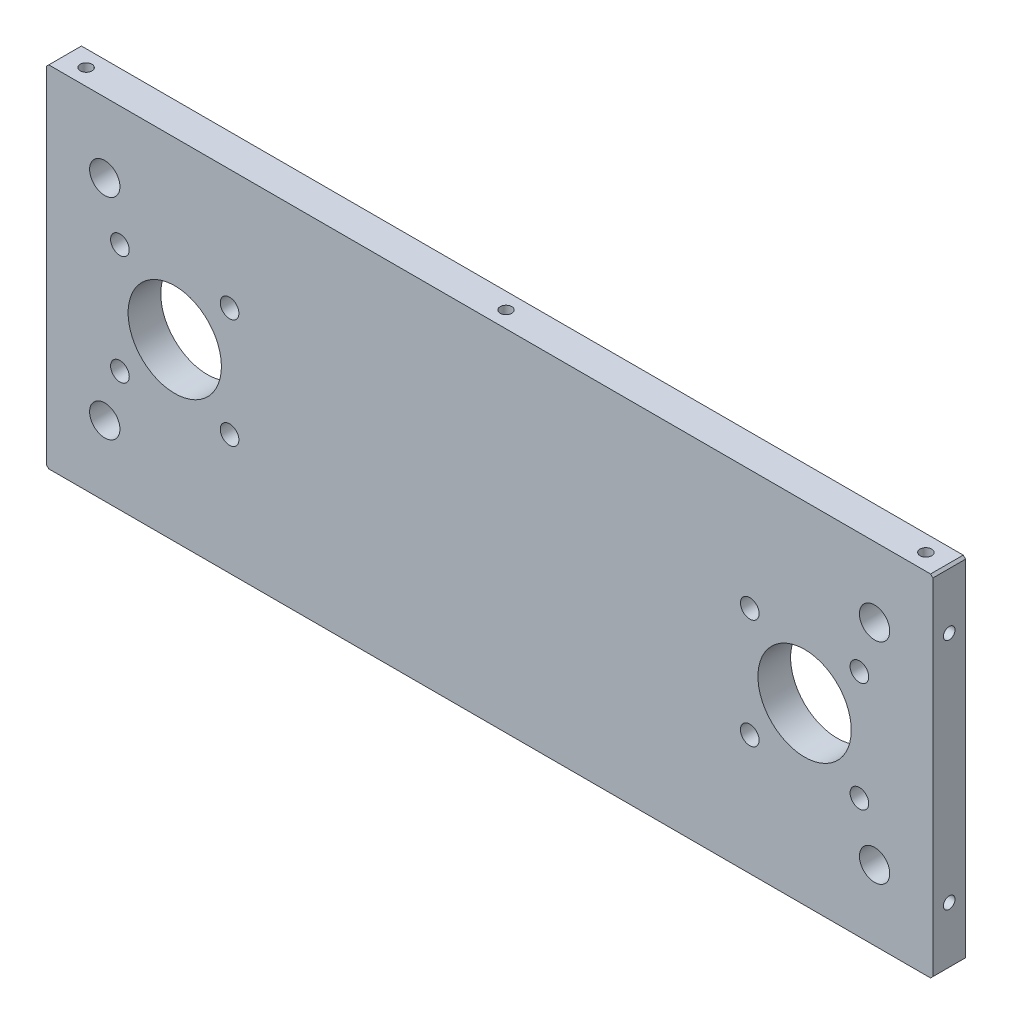
SolidWorks part; units mm, degrees
material "普通碳钢"
ref_plane "Front Plane" through (0, 0, 0) normal (0, 0, 1) x (1, 0, 0)
ref_plane "Top Plane" through (0, 0, 0) normal (0, 1, 0) x (1, 0, 0)
ref_plane "Right Plane" through (0, 0, 0) normal (1, 0, 0) x (0, 0, -1)
sketch "Sketch1" plane through (0, 0, 0) normal (0, 0, 1) x (1, 0, 0)
  line L1 (0, 0) -> (380, 0)
  line L2 (0, 0) -> (0, 150)
  line L3 (0, 150) -> (380, 150)
  line L4 (380, 0) -> (380, 150)
  dimension "D1" = 380
  dimension "D2" = 150
extrude "Boss-Extrude1" add sketch "Sketch1" along normal blind 14
chamfer "Chamfer1" distance 1 angle 45 4 edges at (0, 0, 7) (0, 150, 7) (380, 0, 7) (380, 150, 7)
sketch "Sketch2" plane through (0, 0, 14) normal (0, 0, 1) x (1, 0, 0)
  line L0 (0, 75) -> (55, 75) construction
  line L1 (0, 149) -> (0, 1) construction
  line L2 (55, 75) -> (325, 75) construction
  line L3 (190, 75) -> (190, 150) construction
  line L4 (379, 150) -> (1, 150) construction
  circle A0 centre (55, 75) radius 20
  circle A1 centre (325, 75) radius 20
  dimension "D1" = 40
  dimension "D2" = 270
extrude "Cut-Extrude1" cut sketch "Sketch2" against normal through all
hole_wizard "Ø8.0 (8) Diameter Hole1" positions "3DSketch1" profile "Sketch3" hole size "Ø8.0" standard "GB" end condition through all
sketch3d "3DSketch1"
  line L0 (31.5, 98.5, 14) -> (78.5, 98.5, 14) construction
  line L1 (78.5, 98.5, 14) -> (78.5, 51.5, 14) construction
  line L2 (78.5, 51.5, 14) -> (31.5, 51.5, 14) construction
  line L3 (31.5, 51.5, 14) -> (31.5, 98.5, 14) construction
  line L5 (31.5, 75, 14) -> (55, 75, 14) construction
  line L6 (55, 75, 0) -> (55, 75, 14) construction
  line L7 (55, 75, 14) -> (55, 98.5, 14) construction
  point P0 (31.5, 98.5, 14)
  point P2 (78.5, 98.5, 14)
  point P4 (78.5, 51.5, 14)
  point P6 (31.5, 51.5, 14)
  dimension "D1" = 47
  dimension "D2" = 47
sketch "Sketch3" plane through (31.5, 98.5, 14) normal (1, 0, 0) x (0, -1, 0)
  line L0 (0, 0) -> (0, 14)
  line L1 (0, 14) -> (4, 14)
  line L2 (4, 14) -> (4, 0)
  line L5 (4, 0) -> (0, 0)
  line L11 (0, -6.35) -> (0, 107.95) construction
  dimension "通孔孔直径" = 8
  dimension "通孔孔深度" = 14
pattern_linear "LPattern1" count 2 spacing 270 along (1, 0, 0) of "Ø8.0 (8) Diameter Hole1"
hole_wizard "Ø13.0 (13) Diameter Hole1" positions "3DSketch2" profile "Sketch4" hole size "Ø13.0" standard "GB" end condition through all
sketch3d "3DSketch2"
  line L0 (355, 120, 0) -> (355, 30, 0) construction
  line L1 (355, 30, 0) -> (25, 30, 0) construction
  line L2 (25, 30, 0) -> (25, 120, 0) construction
  line L3 (25, 120, 0) -> (355, 120, 0) construction
  line L5 (355, 75, 0) -> (380, 75, 0) construction
  line L6 (380, 1, 0) -> (380, 149, 0) construction
  line L8 (190, 120, 0) -> (190, 150, 0) construction
  line L9 (379, 150, 0) -> (1, 150, 0) construction
  point P0 (355, 120, 0)
  point P2 (355, 30, 0)
  point P4 (25, 30, 0)
  point P6 (25, 120, 0)
  dimension "D1" = 330
  dimension "D2" = 90
sketch "Sketch4" plane through (355, 120, 0) normal (1, 0, 0) x (0, 1, 0)
  line L0 (0, 0) -> (0, 14)
  line L1 (0, 14) -> (6.5, 14)
  line L2 (6.5, 14) -> (6.5, 0)
  line L5 (6.5, 0) -> (0, 0)
  line L11 (0, -6.35) -> (0, 107.95) construction
  dimension "通孔孔直径" = 13
  dimension "通孔孔深度" = 14
hole_wizard "M6 Tapped Hole1" positions "Sketch5" profile "Sketch6" tap size "M6" standard "GB"
sketch "Sketch5" plane through (0, 0, 0) normal (0, -1, 0) x (-1, 0, 0)
  line L0 (-190, 0) -> (-190, -7) construction
  line L1 (-1, 0) -> (-379, 0) construction
  point P0 (-370, -7)
  point P2 (-190, -7)
  point P4 (-10, -7)
  dimension "D1" = 7
  dimension "D2" = 360
sketch "Sketch6" plane through (370, 0, 7) normal (1, 0, 0) x (0, 0, -1)
  line L0 (0, 0) -> (0, 16.5022)
  line L1 (0, 16.5022) -> (2.5, 15)
  line L2 (2.5, 15) -> (2.5, 0)
  line L5 (2.5, 0) -> (0, 0)
  line L10 (0, 16.5022) -> (-2.5, 15) construction
  line L11 (0, -6.35) -> (0, 107.95) construction
  dimension "螺纹孔钻头直径" = 5
  dimension "螺纹孔钻头深度" = 15
  dimension "导头角度" = 118
cosmetic thread "Cosmetic Thread1" parameters "D1"=12, "D2"=6
cosmetic thread "Cosmetic Thread2" parameters "D1"=12, "D2"=6
cosmetic thread "Cosmetic Thread3" parameters "D1"=12, "D2"=6
hole_wizard "M6 Tapped Hole2" positions "Sketch7" profile "Sketch8" tap size "M6" standard "GB"
sketch "Sketch7" plane through (0, 150, 0) normal (0, 1, 0) x (1, 0, 0)
  point P0 (370, -7)
  point P3 (190, -7)
  point P6 (10, -7)
sketch "Sketch8" plane through (370, 150, 7) normal (1, 0, 0) x (0, 0, 1)
  line L0 (0, 0) -> (0, 16.5022)
  line L1 (0, 16.5022) -> (2.5, 15)
  line L2 (2.5, 15) -> (2.5, 0)
  line L5 (2.5, 0) -> (0, 0)
  line L10 (0, 16.5022) -> (-2.5, 15) construction
  line L11 (0, -6.35) -> (0, 107.95) construction
  dimension "螺纹孔钻头直径" = 5
  dimension "螺纹孔钻头深度" = 15
  dimension "导头角度" = 118
cosmetic thread "Cosmetic Thread4" parameters "D1"=12, "D2"=6
cosmetic thread "Cosmetic Thread5" parameters "D1"=12, "D2"=6
cosmetic thread "Cosmetic Thread6" parameters "D1"=12, "D2"=6
hole_wizard "M6 Tapped Hole3" positions "Sketch9" profile "Sketch10" tap size "M6" standard "GB"
sketch "Sketch9" plane through (380, 0, 0) normal (1, 0, 0) x (0, 0, -1)
  line L0 (-14, 75) -> (0, 75) construction
  line L1 (-14, 1) -> (-14, 149) construction
  line L2 (0, 1) -> (0, 149) construction
  point P0 (-7, 125)
  point P2 (-7, 25)
  dimension "D1" = 100
  dimension "D2" = 7
sketch "Sketch10" plane through (380, 125, 7) normal (0, 1, 0) x (0, 0, -1)
  line L0 (0, 0) -> (0, 16.5022)
  line L1 (0, 16.5022) -> (2.5, 15)
  line L2 (2.5, 15) -> (2.5, 0)
  line L5 (2.5, 0) -> (0, 0)
  line L10 (0, 16.5022) -> (-2.5, 15) construction
  line L11 (0, -6.35) -> (0, 107.95) construction
  dimension "螺纹孔钻头直径" = 5
  dimension "螺纹孔钻头深度" = 15
  dimension "导头角度" = 118
cosmetic thread "Cosmetic Thread7" parameters "D1"=12, "D2"=6
cosmetic thread "Cosmetic Thread8" parameters "D1"=12, "D2"=6
hole_wizard "M6 Tapped Hole4" positions "Sketch11" profile "Sketch12" tap size "M6" standard "GB"
sketch "Sketch11" plane through (0, 0, 0) normal (-1, 0, 0) x (0, 0, 1)
  point P0 (7, 25)
  point P3 (7, 125)
sketch "Sketch12" plane through (0, 25, 7) normal (0, 1, 0) x (0, 0, 1)
  line L0 (0, 0) -> (0, 16.5022)
  line L1 (0, 16.5022) -> (2.5, 15)
  line L2 (2.5, 15) -> (2.5, 0)
  line L5 (2.5, 0) -> (0, 0)
  line L10 (0, 16.5022) -> (-2.5, 15) construction
  line L11 (0, -6.35) -> (0, 107.95) construction
  dimension "螺纹孔钻头直径" = 5
  dimension "螺纹孔钻头深度" = 15
  dimension "导头角度" = 118
cosmetic thread "Cosmetic Thread9" parameters "D1"=12, "D2"=6
cosmetic thread "Cosmetic Thread10" parameters "D1"=12, "D2"=6
